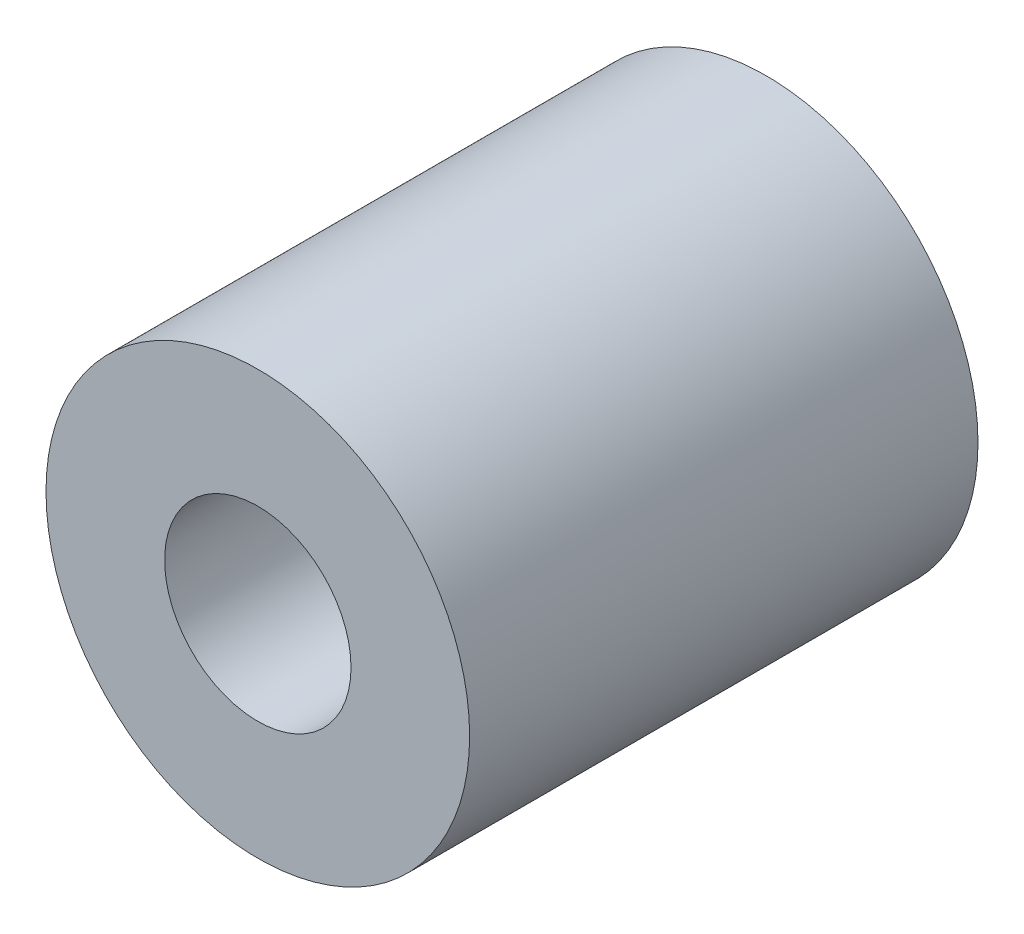
SolidWorks part; units mm, degrees
ref_plane "前视基准面" through (0, 0, 0) normal (0, 0, 1) x (1, 0, 0)
ref_plane "上视基准面" through (0, 0, 0) normal (0, 1, 0) x (1, 0, 0)
ref_plane "右视基准面" through (0, 0, 0) normal (1, 0, 0) x (0, 0, -1)
other "Configuration Table"
sketch "草图1" plane through (0, 0, 0) normal (0, 0, 1) x (1, 0, 0)
  circle A0 centre (0, 0) radius 5
  circle A1 centre (0, 0) radius 2.2
  point P0 (0, 0)
  dimension "D1" = 4.4
  dimension "D2" = 10
extrude "凸台-拉伸1" add sketch "草图1" against normal mid plane 12
